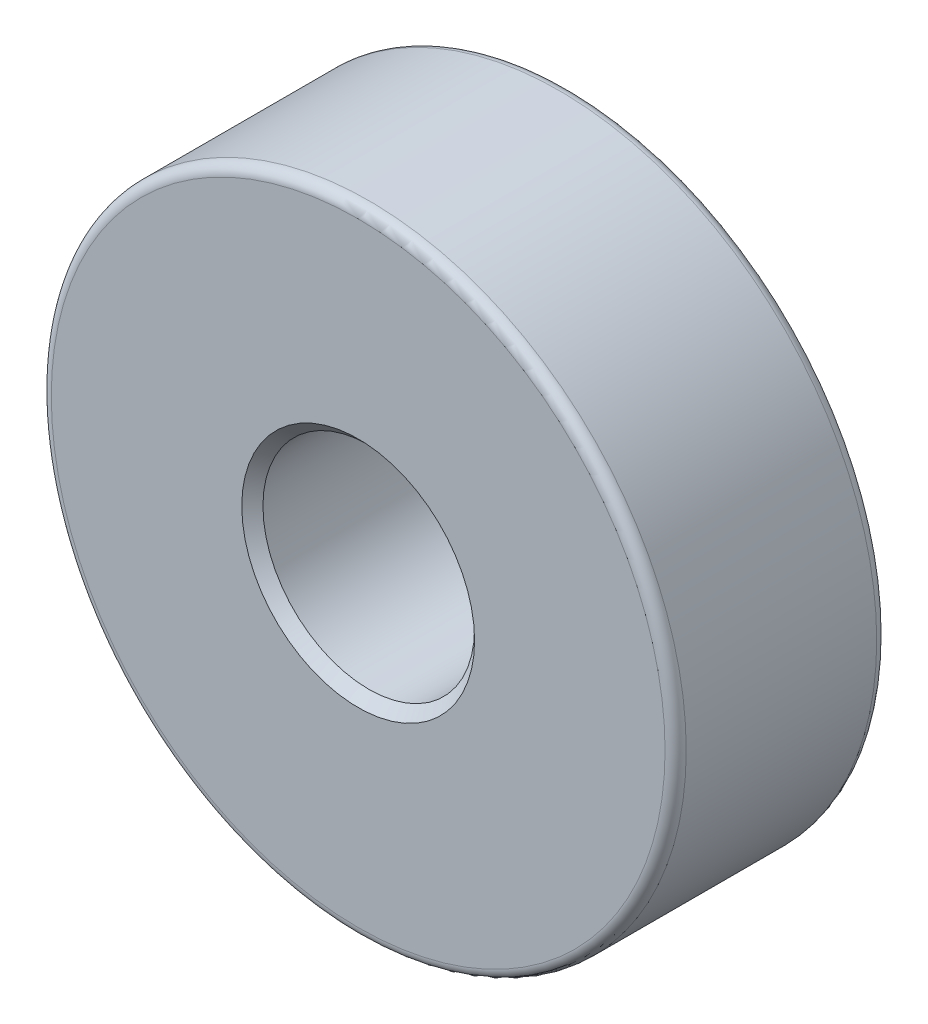
from build123d import *

# Parameters (mm, degrees)
SKETCH_1_R      = 15
SKETCH_1_R_2    = 5
EXTRUDE_1_DEPTH = 10
FILLET_1_R      = 0.5
CHAMFER_1_SIZE  = 0.5


with BuildPart() as part:
    # 草图1 → 凸台-拉伸1 (new body)
    with BuildSketch(Plane.XY):
        Circle(SKETCH_1_R)
        Circle(SKETCH_1_R_2, mode=Mode.SUBTRACT)
    extrude(amount=EXTRUDE_1_DEPTH)

    # 圆角1
    fillet_1_edges = [part.edges().sort_by_distance(p)[0] for p in [
        (-15, 0, 0),
        (-15, 0, 10),
    ]]
    fillet(fillet_1_edges, radius=FILLET_1_R)

    # 倒角1
    chamfer_1_edges = [part.edges().sort_by_distance(p)[0] for p in [
        (-5, 0, 0),
        (-5, 0, 10),
    ]]
    chamfer(chamfer_1_edges, length=CHAMFER_1_SIZE)


solid = part.part
